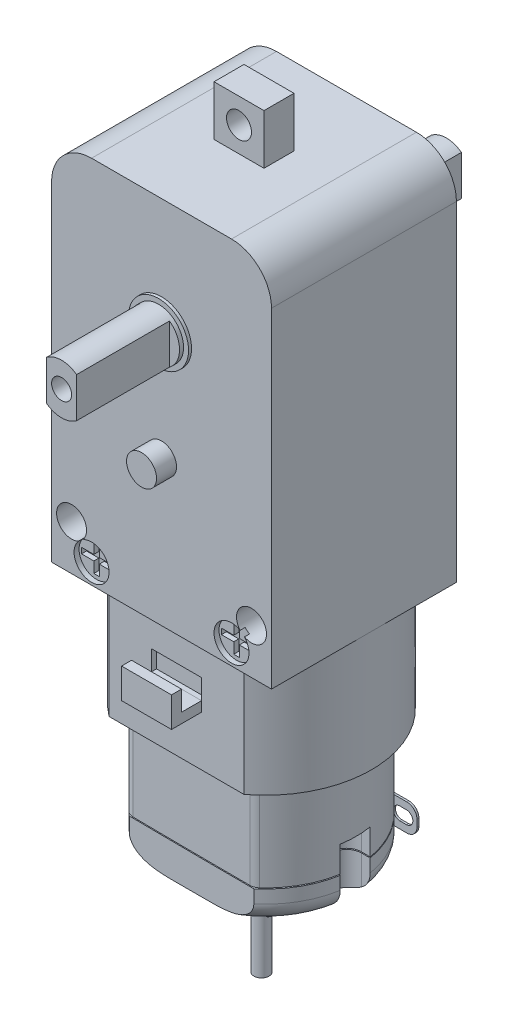
from build123d import *

# Parameters (mm, degrees)
SKETCH1_W                = 22
SKETCH1_H                = 49
BOSS_EXTRUDE1_DEPTH      = 9.25
BOSS_EXTRUDE2_DEPTH      = 1.5
BOSS_EXTRUDE2_DEPTH_BACK = 1.5
SKETCH2_W                = 5
SKETCH2_H                = 10
SKETCH2_R                = 1.25
FILETE1_R                = 4
SKETCH4_R                = 1.5
BOSS_EXTRUDE3_DEPTH      = 2
SKETCH5_OUTSIDE_W        = 36.362
SKETCH5_OUTSIDE_H        = 34.862
CUT_EXTRUDE1_DEPTH       = 12
BOSS_EXTRUDE4_DEPTH      = 15
SKETCH7_W                = 8.294598992
SKETCH7_H                = 0.1
SKETCH8_OUTSIDE_W        = 39.054
SKETCH8_OUTSIDE_H        = 37.554
CUT_EXTRUDE2_DEPTH       = 2.5
FILETE3_R                = 0.5
CUT_EXTRUDE3_DEPTH       = 6
SKETCH10_R               = 0.75
BOSS_EXTRUDE5_DEPTH      = 8
FILETE4_R                = 2
SKETCH11_W               = 8.5
SKETCH11_H               = 3
BOSS_EXTRUDE6_DEPTH      = 2
SKETCH12_W               = 0.2
SKETCH12_H               = 2.7
BOSS_EXTRUDE7_DEPTH      = 3
SKETCH13_W               = 0.2
SKETCH13_H               = 2.7
BOSS_EXTRUDE8_DEPTH      = 3.5
FILETE5_R                = 1
CUT_EXTRUDE4_DEPTH       = 1
BOSS_EXTRUDE9_DEPTH      = 2.5
BOSS_EXTRUDE9_2_DEPTH    = 2.5
FILETE6_R                = 1
SKETCH17_W               = 5
SKETCH17_H               = 2
CUT_EXTRUDE5_DEPTH       = 0.5
SKETCH18_W               = 5
SKETCH18_H               = 2
CUT_EXTRUDE6_DEPTH       = 0.5
SKETCH19_R               = 1.5
CUT_EXTRUDE7_DEPTH       = 54.286959005
SKETCH20_R               = 1.75
CUT_EXTRUDE8_DEPTH       = 0.5
SKETCH21_W               = 1.230384061
SKETCH21_H               = 0.566581058
SKETCH21_W_2             = 0.548893898
SKETCH21_H_2             = 1.083229888
CUT_EXTRUDE9_DEPTH       = 0.5
SKETCH23_R               = 2.5
BOSS_EXTRUDE10_DEPTH     = 10
SKETCH24_R               = 3
SKETCH24_R_2             = 2.5
BOSS_EXTRUDE11_DEPTH     = 0.3
SKETCH25_R               = 2.5
BOSS_EXTRUDE12_DEPTH     = 10
SKETCH26_R               = 3
SKETCH26_R_2             = 2.5
BOSS_EXTRUDE13_DEPTH     = 0.3
SKETCH27_OUTSIDE_W       = 41.772
SKETCH27_OUTSIDE_H       = 96.772
SKETCH27_OUTSIDE_W_2     = 3
SKETCH27_OUTSIDE_H_2     = 11.242451544
SKETCH27_OUTSIDE_R       = 1
CUT_EXTRUDE10_DEPTH      = 9.3
SKETCH28_OUTSIDE_W       = 41.772
SKETCH28_OUTSIDE_H       = 96.772
SKETCH28_OUTSIDE_W_2     = 3
SKETCH28_OUTSIDE_H_2     = 11.242451544
SKETCH28_OUTSIDE_R       = 1
CUT_EXTRUDE11_DEPTH      = 9.3


with BuildPart() as part:
    # Sketch1 → Boss-Extrude1 (new, symmetric)
    with BuildSketch(Plane.XY):
        Rectangle(SKETCH1_W, SKETCH1_H)
    extrude(amount=BOSS_EXTRUDE1_DEPTH, both=True)

    # Sketch2 → Boss-Extrude2 (add, two sides: drawn at the far end of the back side and taken through both)
    with BuildSketch(Plane.XY.offset(-BOSS_EXTRUDE2_DEPTH_BACK)):
        with Locations((0, 24.5)):
            Rectangle(SKETCH2_W, SKETCH2_H)
        with Locations((0, 27)):
            Circle(SKETCH2_R, mode=Mode.SUBTRACT)
    extrude(amount=BOSS_EXTRUDE2_DEPTH + BOSS_EXTRUDE2_DEPTH_BACK)

    # Filete1
    filete1_edges = [part.edges().sort_by_distance(p)[0] for p in [
        (-11, 24.5, 0),
        (11, 24.5, 0),
    ]]
    fillet(filete1_edges, radius=FILETE1_R)

    # Sketch4 → Boss-Extrude3 (add)
    with BuildSketch(Plane.XY.offset(9.25)):
        with Locations((0, 2)):
            Circle(SKETCH4_R)
    extrude(amount=BOSS_EXTRUDE3_DEPTH)

    # Sketch5 outside → Cut-Extrude1 (cut)
    with BuildSketch(Plane.XZ.offset(24.5)):
        with Locations((0, 1)):
            Rectangle(SKETCH5_OUTSIDE_W, SKETCH5_OUTSIDE_H)
        with BuildLine():
            Line((-6.75, 7.75), (6.75, 7.75))
            ThreePointArc((6.75, 7.75), (9.878288904, 4.001644452), (11, -0.75))
            ThreePointArc((11, -0.75), (9.878288904, -5.501644452), (6.75, -9.25))
            Line((6.75, -9.25), (-6.75, -9.25))
            ThreePointArc((-6.75, -9.25), (-9.878288904, -5.501644452), (-11, -0.75))
            ThreePointArc((-11, -0.75), (-9.878288904, 4.001644452), (-6.75, 7.75))
        make_face(mode=Mode.SUBTRACT)
    extrude(amount=-CUT_EXTRUDE1_DEPTH, mode=Mode.SUBTRACT)

    # Sketch6 → Boss-Extrude4 (add)
    with BuildSketch(Plane.XZ.offset(24.5)):
        with BuildLine():
            Line((-6.228684737, -7.75), (6.228684737, -7.75))
            ThreePointArc((6.228684737, -7.75), (9.5, -0.75), (6.228684737, 6.25))
            Line((6.228684737, 6.25), (-6.228684737, 6.25))
            ThreePointArc((-6.228684737, 6.25), (-9.5, -0.75), (-6.228684737, -7.75))
        make_face()
    extrude(amount=BOSS_EXTRUDE4_DEPTH)

    # Sketch7 → Cut-Revolve1 (revolve, cut)
    with BuildSketch(Plane.XY, mode=Mode.PRIVATE) as cut_revolve1_sk:
        with Locations((9.5, -33.65)):
            Rectangle(SKETCH7_W, SKETCH7_H)
    revolve(cut_revolve1_sk.sketch.rotate(Axis((0, 0, 0), (-0.006567406948697803, -0.9999784343504465, 0)), 180), axis=Axis((0, 0, 0), (-0.006567406948697803, -0.9999784343504465, 0)), mode=Mode.SUBTRACT)

    # Sketch8 outside → Cut-Extrude2 (cut)
    with BuildSketch(Plane.XZ.offset(39.5)):
        with Locations((0, 1)):
            Rectangle(SKETCH8_OUTSIDE_W, SKETCH8_OUTSIDE_H)
        with BuildLine():
            Line((-3.741657387, 2.5), (3.741657387, 2.5))
            ThreePointArc((3.741657387, 2.5), (0, -4.5), (-3.741657387, 2.5))
        make_face(mode=Mode.SUBTRACT)
    extrude(amount=-CUT_EXTRUDE2_DEPTH, mode=Mode.SUBTRACT)

    # Filete3
    filete3_edges = [part.edges().sort_by_distance(p)[0] for p in [
        (0, -39.5, -4.5),
        (0, -39.5, 2.5),
    ]]
    fillet(filete3_edges, radius=FILETE3_R)

    # Sketch9 → Cut-Extrude3 (cut)
    with BuildSketch(Plane.XZ.offset(37)):
        with BuildLine():
            Line((-10.5, 0.75), (-8.5, 0.75))
            ThreePointArc((-8.5, 0.75), (-7, -0.75), (-8.5, -2.25))
            Line((-8.5, -2.25), (-10.5, -2.25))
            ThreePointArc((-10.5, -2.25), (-12, -0.75), (-10.5, 0.75))
        make_face()
        with BuildLine():
            Line((10.5, -2.25), (8.5, -2.25))
            ThreePointArc((8.5, -2.25), (7, -0.75), (8.5, 0.75))
            Line((8.5, 0.75), (10.5, 0.75))
            ThreePointArc((10.5, 0.75), (12, -0.75), (10.5, -2.25))
        make_face()
    extrude(amount=-CUT_EXTRUDE3_DEPTH, mode=Mode.SUBTRACT)

    # Filete4
    filete4_edges = [part.edges().sort_by_distance(p)[0] for p in [
        (8.295033735, -37, 3.781963222),
        (8.295033735, -37, -5.281963222),
        (-8.295033735, -37, -5.281963222),
        (-8.295033735, -37, 3.781963222),
    ]]
    fillet(filete4_edges, radius=FILETE4_R)



with BuildPart() as body_2:
    # Sketch10 → Boss-Extrude5 (new body)
    with BuildSketch(Plane.XZ.offset(39.5)):
        with Locations(Location((0, -0.75, 0), (0, 0, 270))):
            Circle(SKETCH10_R)
    extrude(amount=BOSS_EXTRUDE5_DEPTH)


with BuildPart() as body_3:
    # Sketch11 → Boss-Extrude6 (new body)
    with BuildSketch(Plane(origin=(0, 0, -7.75), x_dir=(-1, 0, 0), z_dir=(0, 0, -1))):
        with Locations((0, -35.150533282)):
            Rectangle(SKETCH11_W, SKETCH11_H)
    extrude(amount=BOSS_EXTRUDE6_DEPTH)


with BuildPart() as part_1:
    add(part.part)

    add(body_3.part)  # Boss-Extrude7 merges body 3
    # Sketch12 → Boss-Extrude7 (add)
    with BuildSketch(Plane(origin=(4.25, 0, 0), x_dir=(0, 0, -1), z_dir=(1, 0, 0))):
        with Locations((9.15, -35.150533282)):
            Rectangle(SKETCH12_W, SKETCH12_H)
    extrude(amount=BOSS_EXTRUDE7_DEPTH)

    # Sketch13 → Boss-Extrude8 (add)
    with BuildSketch(Plane.ZY.offset(4.25)):
        with Locations((-9.15, -35.150533282)):
            Rectangle(SKETCH13_W, SKETCH13_H)
    extrude(amount=BOSS_EXTRUDE8_DEPTH)

    # Filete5
    filete5_edges = [part_1.edges().sort_by_distance(p)[0] for p in [
        (7.25, -33.800533282, -9.15),
        (7.25, -36.500533282, -9.15),
        (-7.75, -36.500533282, -9.15),
        (-7.75, -33.800533282, -9.15),
    ]]
    fillet(filete5_edges, radius=FILETE5_R)

    # Sketch14 → Cut-Extrude4 (cut)
    with BuildSketch(Plane(origin=(0, 0, -9.25), x_dir=(-1, 0, 0), z_dir=(0, 0, -1))):
        with BuildLine():
            Line((-6.199040945, -34.507920667), (-5.537235477, -34.507920667))
            ThreePointArc((-5.537235477, -34.507920667), (-4.894622862, -35.150533282), (-5.537235477, -35.793145898))
            Line((-5.537235477, -35.793145898), (-6.199040945, -35.793145898))
            ThreePointArc((-6.199040945, -35.793145898), (-6.841653561, -35.150533282), (-6.199040945, -34.507920667))
        make_face()
        with BuildLine():
            Line((6.199040945, -34.507920667), (5.537235477, -34.507920667))
            ThreePointArc((5.537235477, -34.507920667), (4.894622862, -35.150533282), (5.537235477, -35.793145898))
            Line((5.537235477, -35.793145898), (6.199040945, -35.793145898))
            ThreePointArc((6.199040945, -35.793145898), (6.841653561, -35.150533282), (6.199040945, -34.507920667))
        make_face()
    extrude(amount=-CUT_EXTRUDE4_DEPTH, mode=Mode.SUBTRACT)

    # Filete6
    filete6_edges = [part_1.edges().sort_by_distance(p)[0] for p in [
        (-6.228684737, -29.001800875, 6.25),
        (6.228684737, -29.041686905, 6.25),
        (-6.228684737, -28.998068352, -7.75),
        (6.228684737, -29.038069499, -7.75),
    ]]
    fillet(filete6_edges, radius=FILETE6_R)

    # Sketch17 → Cut-Extrude5 (cut)
    with BuildSketch(Plane(origin=(0, 0, -9.25), x_dir=(-1, 0, 0), z_dir=(0, 0, -1))):
        with Locations((0, -17.5)):
            Rectangle(SKETCH17_W, SKETCH17_H)
    extrude(amount=-CUT_EXTRUDE5_DEPTH, mode=Mode.SUBTRACT)

    # Sketch18 → Cut-Extrude6 (cut)
    with BuildSketch(Plane.XY.offset(7.75)):
        with Locations((0, -17.5)):
            Rectangle(SKETCH18_W, SKETCH18_H)
    extrude(amount=-CUT_EXTRUDE6_DEPTH, mode=Mode.SUBTRACT)

    # Sketch19 → Cut-Extrude7 (cut, through all)
    with BuildSketch(Plane.XY.offset(9.25)):
        with Locations((-9, -8)):
            Circle(SKETCH19_R)
        with Locations((9, -8)):
            Circle(SKETCH19_R)
    extrude(amount=-CUT_EXTRUDE7_DEPTH, mode=Mode.SUBTRACT)

    # Sketch20 → Cut-Extrude8 (cut)
    with BuildSketch(Plane.XY.offset(9.25)):
        with Locations((-7, -10.5)):
            Circle(SKETCH20_R)
        with Locations((7, -10.5)):
            Circle(SKETCH20_R)
    extrude(amount=-CUT_EXTRUDE8_DEPTH, mode=Mode.SUBTRACT)

    # Sketch21 → Cut-Extrude9 (cut)
    with BuildSketch(Plane.XY.offset(8.75)):
        Polygon((-6.725553051, -10.216709471), (-5.49516899, -10.216709471), (-5.49516899, -10.783290529), (-6.725553051, -10.783290529), (-6.725553051, -11.866520417), (-7.274446949, -11.866520417), (-7.274446949, -10.783290529), (-8.50483101, -10.783290529), (-8.50483101, -10.216709471), (-7.274446949, -10.216709471), (-7.274446949, -9.133479583), (-6.725553051, -9.133479583), align=None)
        with Locations((6.110361021, -10.5)):
            Rectangle(SKETCH21_W, SKETCH21_H)
        with Locations((7, -9.675094527)):
            Rectangle(SKETCH21_W_2, SKETCH21_H_2)
        with Locations((7.88963898, -10.5)):
            Rectangle(SKETCH21_W, SKETCH21_H)
        with Locations((7, -11.324905473)):
            Rectangle(SKETCH21_W_2, SKETCH21_H_2)
        with Locations((7, -10.5)):
            Rectangle(SKETCH21_W_2, SKETCH21_H)
    extrude(amount=-CUT_EXTRUDE9_DEPTH, mode=Mode.SUBTRACT)

    # Sketch25 → Boss-Extrude12 (add)
    with BuildSketch(Plane(origin=(0, 0, -9.25), x_dir=(-1, 0, 0), z_dir=(0, 0, -1))):
        with Locations(Location((0, 13, 0), (0, 0, 180))):
            Circle(SKETCH25_R)
    extrude(amount=BOSS_EXTRUDE12_DEPTH)

    # Sketch28 outside → Cut-Extrude11 (cut)
    # profile 1 of 2: a face of its own
    with BuildSketch(Plane(origin=(0, 0, -19.25), x_dir=(-1, 0, 0), z_dir=(0, 0, -1))):
        with Locations((0, -9)):
            Rectangle(SKETCH28_OUTSIDE_W, SKETCH28_OUTSIDE_H)
        with Locations((0, 13)):
            Rectangle(SKETCH28_OUTSIDE_W_2, SKETCH28_OUTSIDE_H_2, mode=Mode.SUBTRACT)
    # profile 2 of 2: a face of its own
    with BuildSketch(Plane(origin=(0, 0, -19.25), x_dir=(-1, 0, 0), z_dir=(0, 0, -1))):
        with Locations(Location((0, 13, 0), (0, 0, 180))):
            Circle(SKETCH28_OUTSIDE_R)
    extrude(amount=-CUT_EXTRUDE11_DEPTH, mode=Mode.SUBTRACT)


with BuildPart() as body_3_2:
    # Sketch16 → Boss-Extrude9 (new, symmetric)
    with BuildSketch(Plane(origin=(0, 0, 0), x_dir=(0, 0, -1), z_dir=(1, 0, 0))):
        Polygon((9.25, -19.5), (12.25, -19.5), (12.25, -16.5), (11.25, -16.5), (11.25, -18.5), (9.25, -18.5), align=None)
    extrude(amount=BOSS_EXTRUDE9_DEPTH, both=True)


with BuildPart() as body_4:
    # Sketch16 → Boss-Extrude9 2 (new, symmetric)
    with BuildSketch(Plane(origin=(0, 0, 0), x_dir=(0, 0, -1), z_dir=(1, 0, 0))):
        Polygon((-7.75, -19.5), (-10.75, -19.5), (-10.75, -16.5), (-9.75, -16.5), (-9.75, -18.5), (-7.75, -18.5), align=None)
    extrude(amount=BOSS_EXTRUDE9_2_DEPTH, both=True)


with BuildPart() as body_5:
    # Sketch23 → Boss-Extrude10 (new body)
    with BuildSketch(Plane.XY.offset(9.25)):
        with Locations((0, 13)):
            Circle(SKETCH23_R)
    extrude(amount=BOSS_EXTRUDE10_DEPTH)

    # Sketch27 outside → Cut-Extrude10 (cut)
    # profile 1 of 2: a face of its own
    with BuildSketch(Plane.XY.offset(19.25)):
        with Locations((0, -9)):
            Rectangle(SKETCH27_OUTSIDE_W, SKETCH27_OUTSIDE_H)
        with Locations((0, 13)):
            Rectangle(SKETCH27_OUTSIDE_W_2, SKETCH27_OUTSIDE_H_2, mode=Mode.SUBTRACT)
    # profile 2 of 2: a face of its own
    with BuildSketch(Plane.XY.offset(19.25)):
        with Locations((0, 13)):
            Circle(SKETCH27_OUTSIDE_R)
    extrude(amount=-CUT_EXTRUDE10_DEPTH, mode=Mode.SUBTRACT)


with BuildPart() as body_6:
    # Sketch24 → Boss-Extrude11 (new body)
    with BuildSketch(Plane.XY.offset(9.25)):
        with Locations((0, 13)):
            Circle(SKETCH24_R)
        with Locations((0, 13)):
            Circle(SKETCH24_R_2, mode=Mode.SUBTRACT)
    extrude(amount=BOSS_EXTRUDE11_DEPTH)


with BuildPart() as body_7:
    # Sketch26 → Boss-Extrude13 (new body)
    with BuildSketch(Plane(origin=(0, 0, -9.25), x_dir=(-1, 0, 0), z_dir=(0, 0, -1))):
        with Locations((0, 13)):
            Circle(SKETCH26_R)
        with Locations((0, 13)):
            Circle(SKETCH26_R_2, mode=Mode.SUBTRACT)
    extrude(amount=BOSS_EXTRUDE13_DEPTH)


solid = Compound([body_2.part, part_1.part, body_3_2.part, body_4.part, body_5.part, body_6.part, body_7.part])
